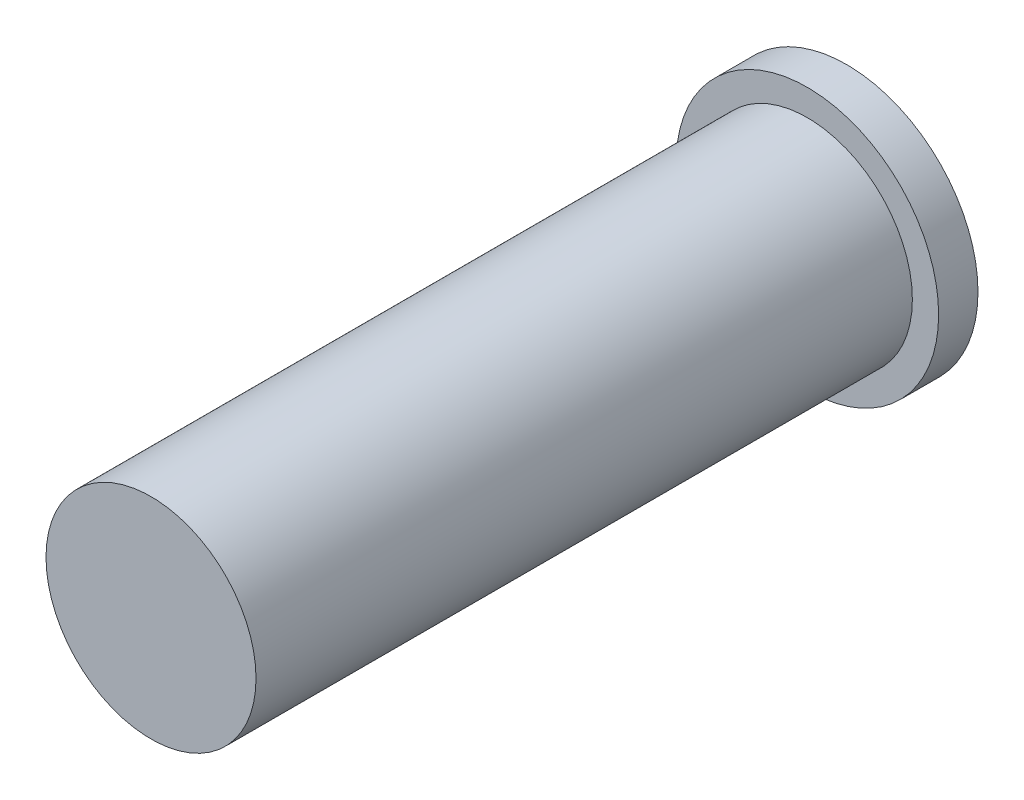
from build123d import *

# Parameters (mm, degrees)
SKETCH_1_R      = 5
EXTRUDE_1_DEPTH = 1.5
SKETCH_2_R      = 4
EXTRUDE_2_DEPTH = 25


with BuildPart() as part:
    # 草图1 → 凸台-拉伸1 (new body)
    with BuildSketch(Plane.XY):
        Circle(SKETCH_1_R)
    extrude(amount=EXTRUDE_1_DEPTH)

    # 草图2 → 凸台-拉伸2 (add)
    with BuildSketch(Plane.XY.offset(1.5)):
        Circle(SKETCH_2_R)
    extrude(amount=EXTRUDE_2_DEPTH)


solid = part.part
